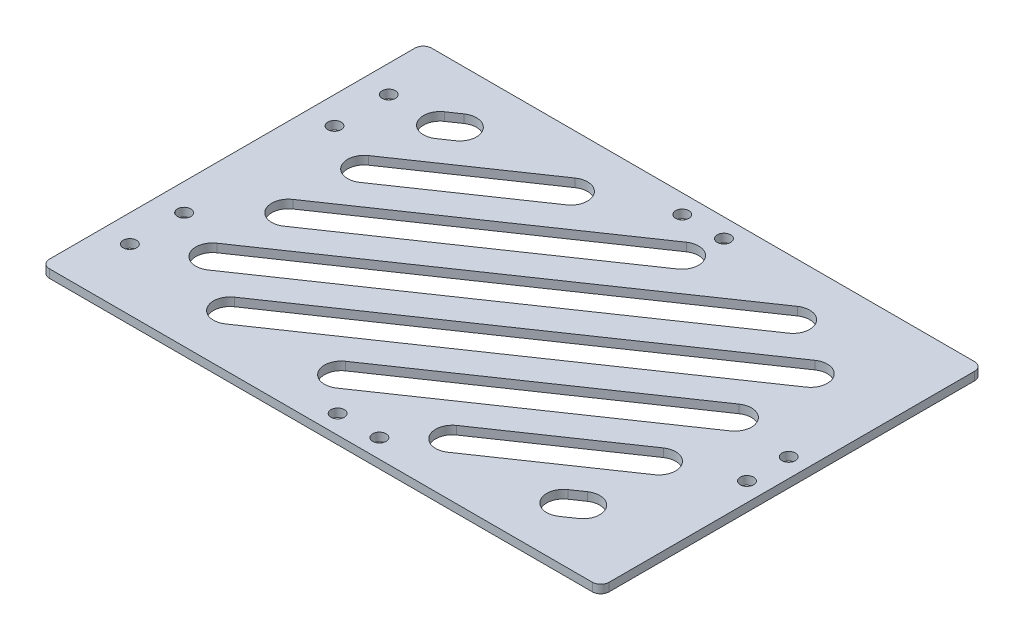
SolidWorks part; units mm, degrees
material "Thornel Mat VMA"
ref_plane "前视基准面" through (0, 0, 0) normal (0, 0, 1) x (1, 0, 0)
ref_plane "上视基准面" through (0, 0, 0) normal (0, 1, 0) x (1, 0, 0)
ref_plane "右视基准面" through (0, 0, 0) normal (1, 0, 0) x (0, 0, -1)
sketch "草图1" plane through (0, 0, 0) normal (0, 1, 0) x (1, 0, 0)
  line L0 (-66, 0) -> (68, 0) construction
  line L1 (-66, 45.75) -> (68, 45.75)
  line L2 (-66, 45.75) -> (-66, -45.75)
  line L3 (-66, -45.75) -> (68, -45.75)
  line L4 (68, 45.75) -> (68, -45.75)
  line L5 (0, 45.75) -> (0, -45.75) construction
  line L6 (-59.5, 31) -> (-59.5, 18) construction
  line L7 (-59.5, -31) -> (-59.5, -18) construction
  line L9 (63.5, 3.75) -> (63.5, -6.25) construction
  line L11 (0.5, -41.25) -> (10.5, -41.25) construction
  line L12 (0.5, 41.25) -> (10.5, 41.25) construction
  circle A0 centre (-59.5, 31) radius 1.6
  circle A1 centre (-59.5, 18) radius 1.6
  circle A2 centre (-59.5, -18) radius 1.6
  circle A3 centre (-59.5, -31) radius 1.6
  circle A6 centre (63.5, 3.75) radius 1.6
  circle A7 centre (63.5, -6.25) radius 1.6
  circle A10 centre (0.5, -41.25) radius 1.6
  circle A11 centre (10.5, -41.25) radius 1.6
  circle A12 centre (10.5, 41.25) radius 1.6
  circle A13 centre (0.5, 41.25) radius 1.6
  point P10 (-66, 0)
  dimension "D1" = 3.2
  dimension "D8" = 4.5
  dimension "D9" = 10
  dimension "D12" = 4.5
  dimension "D10" = 3.2
  dimension "D2" = 13
  dimension "D3" = 68
  dimension "D4" = 66
  dimension "D5" = 91.5
  dimension "D6" = 36
  dimension "D7" = 6.5
  dimension "D11" = 39.5
  dimension "D15" = 57.5
extrude "凸台-拉伸1" add sketch "草图1" along normal blind 2
sketch "队徽" [suppressed] plane through (0, 2, 0) normal (0, 1, 0) x (1, 0, 0)
  line L0 (-25, 38) -> (-25, -22) construction
  line L1 (-12.515, 33.7) -> (-12.515, 35.2787)
  line L2 (-37.485, 33.7) -> (-37.485, 35.2787)
  line L3 (-33.13, 16.8019) -> (-33.13, 11.5819)
  line L4 (-33.13, 11.5819) -> (-34.702, 9.9305)
  line L5 (-34.702, 9.9305) -> (-36.3011, 4.7584)
  line L6 (-33.4579, 3.2225) -> (-31.1856, 10.5724)
  line L7 (-16.5421, 3.2225) -> (-18.8144, 10.5724)
  line L8 (-17.5104, 17.0865) -> (-13.6989, 4.7584)
  line L9 (-21.0663, 32.392) -> (-19.6973, 32.769)
  line L10 (-19.6973, 32.769) -> (-18.0096, 33.5704)
  line L11 (-18.0096, 33.5704) -> (-17.8613, 32.2487)
  line L12 (-18.4024, 35.9034) -> (-17.7524, 35.7605)
  line L13 (-6.1254, -12) -> (-2.6393, -12)
  line L14 (-43.8746, -12) -> (-47.3607, -12)
  arc A0 (-16.6314, -20.8091) -> (-2.6393, -12) centre (-25, 8) ccw
  arc A2 (-33.3686, -20.8091) -> (-33.13, 16.8019) centre (-24.3625, -2.06) cw
  arc A3 (-16.6314, -20.8091) -> (-17.5104, 17.0865) centre (-25.6375, -2.06) ccw
  arc A4 (-19.8705, 26.2753) -> (-12.515, 33.7) centre (-19.94, 33.7) ccw
  arc A5 (-30.1295, 26.2753) -> (-37.485, 33.7) centre (-30.06, 33.7) cw
  arc A6 (-47.3607, -12) -> (-33.3686, -20.8091) centre (-25, 8) ccw
  arc A7 (-36.3011, 4.7584) -> (-33.4579, 3.2225) centre (-25, 22.28) ccw
  arc A9 (-32.1188, 2.6829) -> (-31.1856, 10.5724) centre (-66.67, 10.77) ccw
  arc A10 (-32.1188, 2.6829) -> (-29.0372, 1.8246) centre (-25, 22.28) ccw
  arc A12 (-27.4096, 1.5697) -> (-27.9405, 8.9327) centre (-66.67, 2.44) ccw
  arc A13 (-29.0372, 1.8246) -> (-27.9405, 8.9327) centre (-66.67, 11.27) ccw
  arc A14 (-27.4096, 1.5697) -> (-22.5904, 1.5697) centre (-25, 22.28) ccw
  arc A15 (-22.5904, 1.5697) -> (-22.0595, 8.9327) centre (16.67, 2.44) cw
  arc A16 (-20.9628, 1.8246) -> (-22.0595, 8.9327) centre (16.67, 11.27) cw
  arc A17 (-30.1295, 26.2753) -> (-28.9744, 32.0412) centre (-66.7, 36.6) ccw
  arc A18 (-17.8812, 2.6829) -> (-18.8144, 10.5724) centre (16.67, 10.77) cw
  arc A19 (-19.8705, 26.2753) -> (-21.0663, 32.392) centre (16.7, 36.6) cw
  arc A20 (-20.9628, 1.8246) -> (-17.8812, 2.6829) centre (-25, 22.28) ccw
  arc A21 (-16.5421, 3.2225) -> (-13.6989, 4.7584) centre (-25, 22.28) ccw
  arc A22 (-20.8, 36.4498) -> (-31.4255, 34.2262) centre (-21.93, 15.35) ccw
  arc A23 (-16.5042, 35.0804) -> (-17.7524, 35.7605) centre (-18.3, 33.27) ccw
  arc A25 (-17.8613, 32.2487) -> (-16.5042, 35.0804) centre (-18.3, 34.2) ccw
  arc A29 (-6.1077, 27.9833) -> (-12.515, 35.2787) centre (-17.46, 24.4743) ccw
  arc A30 (-2.2672, 23.4748) -> (-0.7491, 25.6605) centre (-25, 40.8837) ccw
  arc A31 (-6.1077, 27.9833) -> (-5.5019, 30.7996) centre (-25, 33.5203) ccw
  arc A32 (-2.2672, 23.4748) -> (-5.5019, 30.7996) centre (-11.5161, 23.767) ccw
  arc A33 (1.6644, 14.7277) -> (3.8374, 16.2708) centre (-25, 54.5789) ccw
  arc A34 (1.6644, 14.7277) -> (-0.7491, 25.6605) centre (-12.0455, 17.434) ccw
  arc A35 (2.163, 3.7077) -> (4.8783, 5.3) centre (-25, 53.1378) ccw
  arc A36 (2.163, 3.7077) -> (3.8374, 16.2708) centre (-11.3811, 11.906) ccw
  arc A37 (-1.1678, -5.7213) -> (1.8513, -5.3793) centre (-25, 218.1341) ccw
  arc A38 (-1.1678, -5.7213) -> (4.8783, 5.3) centre (-10.7675, 6.7139) ccw
  arc A40 (-6.1254, -12) -> (1.8513, -5.3793) centre (-9.635, 0.344) ccw
  circle A41 centre (-25, 8) radius 27.5 construction
  arc A42 (-43.8923, 27.9833) -> (-44.4981, 30.7996) centre (-25, 33.5203) cw
  arc A43 (-43.8923, 27.9833) -> (-37.485, 35.2787) centre (-32.54, 24.4743) cw
  arc A44 (-47.7328, 23.4748) -> (-44.4981, 30.7996) centre (-38.4839, 23.767) cw
  arc A45 (-47.7328, 23.4748) -> (-49.2509, 25.6605) centre (-25, 40.8837) cw
  arc A46 (-51.6644, 14.7277) -> (-49.2509, 25.6605) centre (-37.9545, 17.434) cw
  arc A47 (-51.6644, 14.7277) -> (-53.8374, 16.2708) centre (-25, 54.5789) cw
  arc A48 (-52.163, 3.7077) -> (-53.8374, 16.2708) centre (-38.6189, 11.906) cw
  arc A49 (-52.163, 3.7077) -> (-54.8783, 5.3) centre (-25, 53.1378) cw
  arc A50 (-48.8322, -5.7213) -> (-54.8783, 5.3) centre (-39.2325, 6.7139) cw
  arc A51 (-48.8322, -5.7213) -> (-51.8513, -5.3793) centre (-25, 218.1341) cw
  arc A52 (-43.8746, -12) -> (-51.8513, -5.3793) centre (-40.365, 0.344) cw
  arc A53 (-28.9744, 32.0412) -> (-31.4255, 34.2262) centre (-30.96, 32.2812) ccw
  spline S0 degree 3 poles (-20.8, 36.4498) (-20.2858, 35.8279) (-18.8685, 36.0059) (-18.4024, 35.9034) knots 0 0 0 0 1 1 1 1
  spline S1 degree 3 poles (-22.2858, 34.0584) (-22.7796, 35.9592) (-21.5435, 34.6039) (-20.1915, 35.1653) (-20.9556, 33.6368) (-22.2858, 34.0584) (-22.7796, 35.9592) (-21.5435, 34.6039) knots -0.60913 -0.442651 -0.194324 0 0.241967 0.39087 0.557349 0.805676 1 1.241967 1.39087 1.557349 only from (-22.5, 35.3861) to (-22.5, 35.3861)
  dimension "D1" = 60
  dimension "D2" = 20.8
  dimension "D5" = 25.7
  dimension "D7" = 7.425
  dimension "D8" = 41.7
  dimension "D16" = 35.485
  dimension "D19" = 39.27
  dimension "D21" = 0.5
  dimension "D22" = 38.8
  dimension "D23" = 41.7
  dimension "D25" = 55
  dimension "D26" = 7.35
  dimension "D28" = 21.13
  dimension "D29" = 25.27
  dimension "D31" = 0.93
  dimension "D32" = 2
  dimension "D33" = 5.1
  dimension "D41" = 8
  dimension "D42" = 9.59
  dimension "D44" = 7
  dimension "D46" = 10
  dimension "D48" = 20
  dimension "D49" = 11.1
  dimension "D43" = 11.02
  dimension "D47" = 8
  dimension "D52" = 38
  dimension "D57" = 2
  dimension "D3" = 10.06
  dimension "D4" = 1.275
  dimension "D6" = 10.12
  dimension "D9" = 14.28
  dimension "D10" = 8.13
  dimension "D11" = 5.22
  dimension "D12" = 136.41
  dimension "D13" = 2.28
  dimension "D14" = 17.18
  dimension "D15" = 3.17
  dimension "D17" = 41.67
  dimension "D18" = 2.77
  dimension "D20" = 8.33
  dimension "D24" = 28.6
  dimension "D27" = 3.07
  dimension "D30" = 6.7
  dimension "D34" = 74.6
  dimension "D35" = 1.42
  dimension "D36" = 170
  dimension "D37" = 71
  dimension "D38" = 1.33
  dimension "D39" = 0.65
  dimension "D40" = 77.6
  dimension "D45" = 7.54
  dimension "D50" = 11.02
  dimension "D51" = 10.45
  dimension "D53" = 4.8
  dimension "D54" = 28.5
  dimension "D55" = 4.2
  dimension "D56" = 90
  dimension "D58" = 5.96
  dimension "D59" = 2.5
  dimension "D60" = 2
  dimension "D61" = 0.5
  dimension "D62" = 1.2
  dimension "D63" = 0.3
  dimension "D64" = 0.4
  dimension "D65" = 1
  dimension "D66" = 0.8
  dimension "D67" = 8
  dimension "D68" = 25
sketch "草图4" [suppressed] plane through (0, 2, 0) normal (0, 1, 0) x (1, 0, 0)
  line L0 (-25, 42) -> (-25, -26) construction
  line L3 (-27.5, 41.908) -> (-27.5, 35.7326)
  line L8 (-22.5, 41.908) -> (-22.5, 36.4723)
  line L9 (6.4758, 20.8558) -> (1.7989, 19.3361)
  line L10 (8.0209, 16.1005) -> (4.1747, 14.8508)
  line L11 (-3.0469, -17.9627) -> (-5.4052, -14.7166)
  line L12 (-7.0919, -20.9016) -> (-9.4503, -17.6556)
  line L13 (-42.9081, -20.9016) -> (-40.5497, -17.6556)
  line L42 (-46.9531, -17.9627) -> (-44.5948, -14.7166)
  line L43 (-58.0209, 16.1005) -> (-54.1747, 14.8508)
  line L44 (-56.4758, 20.8558) -> (-51.7989, 19.3361)
  line L45 (-43.3105, 6.5198) -> (-49.4142, 0.4161)
  line L46 (-44.7, 2.3019) -> (-48, -0.9981)
  line L48 (-43.8746, -12) -> (-47.3607, -12)
  line L49 (-33.13, 16.8019) -> (-33.13, 11.5819)
  line L50 (-33.13, 11.5819) -> (-34.702, 9.9305)
  line L51 (-34.702, 9.9305) -> (-36.3011, 4.7584)
  line L52 (-33.4579, 3.2225) -> (-31.1856, 10.5724)
  line L53 (-18.8144, 10.5724) -> (-16.5421, 3.2225)
  line L54 (-13.6989, 4.7584) -> (-17.5104, 17.0865)
  line L55 (-2.6393, -12) -> (-6.1254, -12)
  line L56 (-12.515, 35.2787) -> (-12.515, 33.7)
  line L57 (-21.0663, 32.392) -> (-19.6973, 32.769)
  line L58 (-19.6973, 32.769) -> (-18.0096, 33.5704)
  line L59 (-18.0096, 33.5704) -> (-17.8613, 32.2487)
  line L60 (-17.7524, 35.7605) -> (-18.4024, 35.9034)
  line L61 (-37.485, 33.7) -> (-37.485, 35.2787)
  line L62 (-43.8746, -12) -> (-47.3607, -12)
  line L63 (-33.13, 16.8019) -> (-33.13, 11.5819)
  line L64 (-33.13, 11.5819) -> (-34.702, 9.9305)
  line L65 (-34.702, 9.9305) -> (-36.3011, 4.7584)
  line L66 (-33.4579, 3.2225) -> (-31.1856, 10.5724)
  line L67 (-18.8144, 10.5724) -> (-16.5421, 3.2225)
  line L68 (-13.6989, 4.7584) -> (-17.5104, 17.0865)
  line L69 (-2.6393, -12) -> (-6.1254, -12)
  line L70 (-12.515, 35.2787) -> (-12.515, 33.7)
  line L71 (-21.0663, 32.392) -> (-19.6973, 32.769)
  line L72 (-19.6973, 32.769) -> (-18.0096, 33.5704)
  line L73 (-18.0096, 33.5704) -> (-17.8613, 32.2487)
  line L74 (-17.7524, 35.7605) -> (-18.4024, 35.9034)
  line L75 (-37.485, 33.7) -> (-37.485, 35.2787)
  line L77 (-49.4142, 0.4161) -> (-48, -0.9981)
  line L78 (-44.8311, 21.2627) -> (-36.3458, 29.7479) construction
  line L79 (-54.0846, 8.5198) -> (-50.5029, 8.5198)
  line L80 (-50.5029, 8.5198) -> (-36.2226, 22.8001)
  line L81 (-53.5066, 6.5198) -> (-49.6745, 6.5198)
  line L82 (-49.6745, 6.5198) -> (-34.8084, 21.3859)
  line L83 (-44.5227, 22.9853) -> (-36.8384, 30.6696)
  line L84 (-43.1085, 21.5711) -> (-35.7499, 28.9297)
  arc A6 (-27.5, 41.908) -> (-56.4758, 20.8558) centre (-25, 8) ccw
  arc A7 (-27.5, 35.7326) -> (-31.4255, 34.2262) centre (-21.93, 15.35) ccw
  arc A8 (-42.9081, -20.9016) -> (-7.0919, -20.9016) centre (-25, 8) ccw
  arc A9 (-40.5497, -17.6556) -> (-33.3686, -20.8091) centre (-25, 8) ccw
  arc A10 (-3.0469, -17.9627) -> (8.0209, 16.1005) centre (-25, 8) ccw
  arc A11 (-5.4052, -14.7166) -> (-2.6393, -12) centre (-25, 8) ccw
  arc A12 (6.4758, 20.8558) -> (-22.5, 41.908) centre (-25, 8) ccw
  arc A13 (-58.0209, 16.1005) -> (-46.9531, -17.9627) centre (-25, 8) ccw
  arc A15 (-44.7, 2.3019) -> (-33.3686, -20.8091) centre (-24.3625, -2.06) ccw
  arc A18 (-34.8084, 21.3859) -> (-36.2226, 22.8001) centre (-34.5, 23.1085) ccw
  arc A19 (-53.5066, 6.5198) -> (-52.163, 3.7077) centre (-38.6189, 11.906) ccw
  arc A20 (-44.5227, 22.9853) -> (-43.1085, 21.5711) centre (-44.8311, 21.2627) ccw
  arc A21 (-35.7499, 28.9297) -> (-30.1295, 26.2753) centre (-30.06, 33.7) ccw
  arc A135 (-47.3607, -12) -> (-33.3686, -20.8091) centre (-25, 8) ccw
  arc A136 (-33.13, 16.8019) -> (-33.3686, -20.8091) centre (-24.3625, -2.06) ccw
  arc A137 (-36.3011, 4.7584) -> (-33.4579, 3.2225) centre (-25, 22.28) ccw
  arc A138 (-32.1188, 2.6829) -> (-31.1856, 10.5724) centre (-66.67, 10.77) ccw
  arc A139 (-32.1188, 2.6829) -> (-29.0372, 1.8246) centre (-25, 22.28) ccw
  arc A140 (-29.0372, 1.8246) -> (-27.9405, 8.9327) centre (-66.67, 11.27) ccw
  arc A141 (-27.4096, 1.5697) -> (-27.9405, 8.9327) centre (-66.67, 2.44) ccw
  arc A142 (-27.4096, 1.5697) -> (-22.5904, 1.5697) centre (-25, 22.28) ccw
  arc A143 (-22.0595, 8.9327) -> (-22.5904, 1.5697) centre (16.67, 2.44) ccw
  arc A144 (-22.0595, 8.9327) -> (-20.9628, 1.8246) centre (16.67, 11.27) ccw
  arc A145 (-20.9628, 1.8246) -> (-17.8812, 2.6829) centre (-25, 22.28) ccw
  arc A146 (-18.8144, 10.5724) -> (-17.8812, 2.6829) centre (16.67, 10.77) ccw
  arc A147 (-16.5421, 3.2225) -> (-13.6989, 4.7584) centre (-25, 22.28) ccw
  arc A148 (-16.6314, -20.8091) -> (-17.5104, 17.0865) centre (-25.6375, -2.06) ccw
  arc A149 (-16.6314, -20.8091) -> (-2.6393, -12) centre (-25, 8) ccw
  arc A150 (-6.1254, -12) -> (1.8513, -5.3793) centre (-9.635, 0.344) ccw
  arc A151 (-1.1678, -5.7213) -> (1.8513, -5.3793) centre (-25, 218.1341) ccw
  arc A152 (-1.1678, -5.7213) -> (4.8783, 5.3) centre (-10.7675, 6.7139) ccw
  arc A153 (2.163, 3.7077) -> (4.8783, 5.3) centre (-25, 53.1378) ccw
  arc A154 (2.163, 3.7077) -> (3.8374, 16.2708) centre (-11.3811, 11.906) ccw
  arc A155 (1.6644, 14.7277) -> (3.8374, 16.2708) centre (-25, 54.5789) ccw
  arc A156 (1.6644, 14.7277) -> (-0.7491, 25.6605) centre (-12.0455, 17.434) ccw
  arc A157 (-2.2672, 23.4748) -> (-0.7491, 25.6605) centre (-25, 40.8837) ccw
  arc A158 (-2.2672, 23.4748) -> (-5.5019, 30.7996) centre (-11.5161, 23.767) ccw
  arc A159 (-6.1077, 27.9833) -> (-5.5019, 30.7996) centre (-25, 33.5203) ccw
  arc A160 (-6.1077, 27.9833) -> (-12.515, 35.2787) centre (-17.46, 24.4743) ccw
  arc A161 (-19.8705, 26.2753) -> (-12.515, 33.7) centre (-19.94, 33.7) ccw
  arc A162 (-21.0663, 32.392) -> (-19.8705, 26.2753) centre (16.7, 36.6) ccw
  arc A163 (-17.8613, 32.2487) -> (-16.5042, 35.0804) centre (-18.3, 34.2) ccw
  arc A164 (-16.5042, 35.0804) -> (-17.7524, 35.7605) centre (-18.3, 33.27) ccw
  arc A165 (-20.8, 36.4498) -> (-31.4255, 34.2262) centre (-21.93, 15.35) ccw
  arc A166 (-30.1295, 26.2753) -> (-28.9744, 32.0412) centre (-66.7, 36.6) ccw
  arc A167 (-37.485, 33.7) -> (-30.1295, 26.2753) centre (-30.06, 33.7) ccw
  arc A168 (-37.485, 35.2787) -> (-43.8923, 27.9833) centre (-32.54, 24.4743) ccw
  arc A169 (-44.4981, 30.7996) -> (-43.8923, 27.9833) centre (-25, 33.5203) ccw
  arc A170 (-44.4981, 30.7996) -> (-47.7328, 23.4748) centre (-38.4839, 23.767) ccw
  arc A171 (-49.2509, 25.6605) -> (-47.7328, 23.4748) centre (-25, 40.8837) ccw
  arc A172 (-49.2509, 25.6605) -> (-51.6644, 14.7277) centre (-37.9545, 17.434) ccw
  arc A173 (-53.8374, 16.2708) -> (-51.6644, 14.7277) centre (-25, 54.5789) ccw
  arc A174 (-53.8374, 16.2708) -> (-52.163, 3.7077) centre (-38.6189, 11.906) ccw
  arc A175 (-54.8783, 5.3) -> (-52.163, 3.7077) centre (-25, 53.1378) ccw
  arc A176 (-54.8783, 5.3) -> (-48.8322, -5.7213) centre (-39.2325, 6.7139) ccw
  arc A177 (-51.8513, -5.3793) -> (-48.8322, -5.7213) centre (-25, 218.1341) ccw
  arc A178 (-51.8513, -5.3793) -> (-43.8746, -12) centre (-40.365, 0.344) ccw
  arc A179 (-47.3607, -12) -> (-44.5948, -14.7166) centre (-25, 8) ccw
  arc A180 (-33.13, 16.8019) -> (-43.3105, 6.5198) centre (-24.3625, -2.06) ccw
  arc A181 (-36.3011, 4.7584) -> (-33.4579, 3.2225) centre (-25, 22.28) ccw
  arc A182 (-32.1188, 2.6829) -> (-31.1856, 10.5724) centre (-66.67, 10.77) ccw
  arc A183 (-32.1188, 2.6829) -> (-29.0372, 1.8246) centre (-25, 22.28) ccw
  arc A184 (-29.0372, 1.8246) -> (-27.9405, 8.9327) centre (-66.67, 11.27) ccw
  arc A185 (-27.4096, 1.5697) -> (-27.9405, 8.9327) centre (-66.67, 2.44) ccw
  arc A186 (-27.4096, 1.5697) -> (-22.5904, 1.5697) centre (-25, 22.28) ccw
  arc A187 (-22.0595, 8.9327) -> (-22.5904, 1.5697) centre (16.67, 2.44) ccw
  arc A188 (-22.0595, 8.9327) -> (-20.9628, 1.8246) centre (16.67, 11.27) ccw
  arc A189 (-20.9628, 1.8246) -> (-17.8812, 2.6829) centre (-25, 22.28) ccw
  arc A190 (-18.8144, 10.5724) -> (-17.8812, 2.6829) centre (16.67, 10.77) ccw
  arc A191 (-16.5421, 3.2225) -> (-13.6989, 4.7584) centre (-25, 22.28) ccw
  arc A192 (-16.6314, -20.8091) -> (-17.5104, 17.0865) centre (-25.6375, -2.06) ccw
  arc A193 (-16.6314, -20.8091) -> (-9.4503, -17.6556) centre (-25, 8) ccw
  arc A194 (-6.1254, -12) -> (1.8513, -5.3793) centre (-9.635, 0.344) ccw
  arc A195 (-1.1678, -5.7213) -> (1.8513, -5.3793) centre (-25, 218.1341) ccw
  arc A196 (-1.1678, -5.7213) -> (4.8783, 5.3) centre (-10.7675, 6.7139) ccw
  arc A197 (2.163, 3.7077) -> (4.8783, 5.3) centre (-25, 53.1378) ccw
  arc A198 (2.163, 3.7077) -> (4.1747, 14.8508) centre (-11.3811, 11.906) ccw
  arc A200 (1.7989, 19.3361) -> (-0.7491, 25.6605) centre (-12.0455, 17.434) ccw
  arc A201 (-2.2672, 23.4748) -> (-0.7491, 25.6605) centre (-25, 40.8837) ccw
  arc A202 (-2.2672, 23.4748) -> (-5.5019, 30.7996) centre (-11.5161, 23.767) ccw
  arc A203 (-6.1077, 27.9833) -> (-5.5019, 30.7996) centre (-25, 33.5203) ccw
  arc A204 (-6.1077, 27.9833) -> (-12.515, 35.2787) centre (-17.46, 24.4743) ccw
  arc A205 (-19.8705, 26.2753) -> (-12.515, 33.7) centre (-19.94, 33.7) ccw
  arc A206 (-21.0663, 32.392) -> (-19.8705, 26.2753) centre (16.7, 36.6) ccw
  arc A207 (-17.8613, 32.2487) -> (-16.5042, 35.0804) centre (-18.3, 34.2) ccw
  arc A208 (-16.5042, 35.0804) -> (-17.7524, 35.7605) centre (-18.3, 33.27) ccw
  arc A209 (-20.8, 36.4498) -> (-22.5, 36.4723) centre (-21.93, 15.35) ccw
  arc A210 (-30.1295, 26.2753) -> (-28.9744, 32.0412) centre (-66.7, 36.6) ccw
  arc A211 (-37.485, 33.7) -> (-36.8384, 30.6696) centre (-30.06, 33.7) ccw
  arc A212 (-37.485, 35.2787) -> (-43.8923, 27.9833) centre (-32.54, 24.4743) ccw
  arc A213 (-44.4981, 30.7996) -> (-43.8923, 27.9833) centre (-25, 33.5203) ccw
  arc A214 (-44.4981, 30.7996) -> (-47.7328, 23.4748) centre (-38.4839, 23.767) ccw
  arc A215 (-49.2509, 25.6605) -> (-47.7328, 23.4748) centre (-25, 40.8837) ccw
  arc A216 (-49.2509, 25.6605) -> (-51.7989, 19.3361) centre (-37.9545, 17.434) ccw
  arc A218 (-54.1747, 14.8508) -> (-54.0846, 8.5198) centre (-38.6189, 11.906) ccw
  arc A219 (-54.8783, 5.3) -> (-52.163, 3.7077) centre (-25, 53.1378) ccw
  arc A220 (-54.8783, 5.3) -> (-48.8322, -5.7213) centre (-39.2325, 6.7139) ccw
  arc A221 (-51.8513, -5.3793) -> (-48.8322, -5.7213) centre (-25, 218.1341) ccw
  arc A222 (-51.8513, -5.3793) -> (-43.8746, -12) centre (-40.365, 0.344) ccw
  arc A232 (-28.9744, 32.0412) -> (-31.4255, 34.2262) centre (-30.96, 32.2812) ccw
  arc A233 (-28.9744, 32.0412) -> (-31.4255, 34.2262) centre (-30.96, 32.2812) ccw
  spline S0 degree 3 poles (-21.5435, 34.6039) (-22.7796, 35.9592) (-22.2858, 34.0584) (-20.9556, 33.6368) (-20.1915, 35.1653) (-21.5435, 34.6039) (-22.7796, 35.9592) (-22.2858, 34.0584) knots -0.557349 -0.39087 -0.241967 0 0.194324 0.442651 0.60913 0.758033 1 1.194324 1.442651 1.60913 only from (-22.5, 35.3861) to (-22.5, 35.3861) construction
  spline S1 degree 3 poles (-1772.4748, -924.8076) (1747.4533, 1033.1302) (-1763.0741, -1000.2366) (1663.8646, 1113.8816) knots -9.353839 -9.353839 -9.353839 -9.353839 10.249272 10.249272 10.249272 10.249272 only from (-18.4024, 35.9034) to (-20.8, 36.4498)
  spline S2 degree 3 poles (-18.4024, 35.9034) (-18.8685, 36.0059) (-20.2858, 35.8279) (-20.8, 36.4498) knots 0 0 0 0 1 1 1 1
  spline S3 degree 3 poles (-21.5435, 34.6039) (-22.7796, 35.9592) (-22.2858, 34.0584) (-20.9556, 33.6368) (-20.1915, 35.1653) (-21.5435, 34.6039) (-22.7796, 35.9592) (-22.2858, 34.0584) knots -0.557349 -0.39087 -0.241967 0 0.194324 0.442651 0.60913 0.758033 1 1.194324 1.442651 1.60913 only from (-22.5, 35.3861) to (-22.5, 35.3861)
  point P86 (-25, 8)
  dimension "D2" = 4
  dimension "D4" = 5
  dimension "D5" = 1.75
  dimension "D8" = 2
  dimension "D12" = 2
  dimension "D14" = 1
  dimension "D3" = 5
  dimension "D6" = 2
  dimension "D7" = 45
  dimension "D9" = 4
  dimension "D10" = 19.7
  dimension "D11" = 23
  dimension "D13" = 2
  dimension "D15" = 12
  dimension "D16" = 9.5
  dimension "D17" = 4.5
  dimension "D21" = 8
  dimension "D1" = 0
extrude "切除-拉伸1" [suppressed] cut sketch "草图4" against normal through all contours A210 A233 A7 L3 A6 L44 A216 A215 A214 A213 A212 L75 A211 | S2 L74 A208 A207 L73 L72 L71 A206 A205 L70 A204 A203 A202 A201 A200 L9 A12 L8 A209 | A222 A221 A220 A219 A218 L43 A13 L42 A179 L62 | L0 A186 A185 A184 A183 A182 L66 A181 L65 L64 L63 A180 A9 L13 A8 | A186 L0 A8 L12 A193 A192 L68 A191 L67 A190 A189 A188 A187 | A198 A197 A196 A195 A194 L69 A11 L11 A10 L10 | S3
fillet "R0.5 圆角1" [suppressed] radius 0.5
fillet "R0.5 圆角2" [suppressed] radius 0.5
fillet "R2 圆角3" [suppressed] radius 2
sketch "草图5" plane through (0, 2, 0) normal (0, 1, 0) x (1, 0, 0)
  line L0 (-66, -45.75) -> (68, 45.75) construction
  line L1 (-47, 30.7958) -> (-44.2163, 32.6966) construction
  line L2 (-49.2556, 34.0992) -> (-46.472, 36)
  line L3 (-44.7444, 27.4925) -> (-41.9607, 29.3933)
  line L4 (-47, 12.6324) -> (-17.6163, 32.6966) construction
  line L5 (-49.2556, 15.9358) -> (-19.872, 36)
  line L6 (-44.7444, 9.3291) -> (-15.3607, 29.3933)
  line L7 (-47, -5.531) -> (8.9836, 32.6966) construction
  line L8 (-49.2556, -2.2277) -> (6.728, 36)
  line L9 (-44.7444, -8.8343) -> (11.2393, 29.3933)
  line L10 (-47, -23.6944) -> (35.5836, 32.6966) construction
  line L11 (-49.2556, -20.3911) -> (33.328, 36)
  line L12 (-44.7444, -26.9978) -> (37.8392, 29.3933)
  line L13 (-33.7, -32.7761) -> (48.8836, 23.6149) construction
  line L14 (-66.1164, 45.75) -> (68, -45.8295) construction
  line L15 (-35.9557, -29.4728) -> (46.6279, 26.9183)
  line L16 (-31.4444, -36.0795) -> (51.1392, 20.3116)
  line L17 (-7.1, -32.7761) -> (48.8836, 5.4515) construction
  line L18 (-9.3557, -29.4728) -> (46.6279, 8.7549)
  line L19 (-4.8444, -36.0795) -> (51.1392, 2.1482)
  line L20 (19.4999, -32.7761) -> (48.8836, -12.7119) construction
  line L21 (17.2443, -29.4728) -> (46.6279, -9.4086)
  line L22 (21.7556, -36.0795) -> (51.1392, -16.0153)
  line L23 (46.0999, -32.7761) -> (48.8836, -30.8753) construction
  line L24 (43.8443, -29.4728) -> (46.6279, -27.572)
  line L25 (48.3555, -36.0795) -> (51.1392, -34.1787)
  line L26 (-66, 45.75) -> (68, -45.75) construction
  line L27 (68, 45.75) -> (-66, 45.75) construction
  line L28 (68, -45.75) -> (68, 45.75) construction
  arc A0 (-49.2556, 34.0992) -> (-44.7444, 27.4925) centre (-47, 30.7958) ccw
  arc A1 (-41.9607, 29.3933) -> (-46.472, 36) centre (-44.2163, 32.6966) ccw
  arc A2 (-49.2556, 15.9358) -> (-44.7444, 9.3291) centre (-47, 12.6324) ccw
  arc A3 (-15.3607, 29.3933) -> (-19.872, 36) centre (-17.6163, 32.6966) ccw
  arc A4 (-49.2556, -2.2277) -> (-44.7444, -8.8343) centre (-47, -5.531) ccw
  arc A5 (11.2393, 29.3933) -> (6.728, 36) centre (8.9836, 32.6966) ccw
  arc A6 (-49.2556, -20.3911) -> (-44.7444, -26.9978) centre (-47, -23.6944) ccw
  arc A7 (37.8392, 29.3933) -> (33.328, 36) centre (35.5836, 32.6966) ccw
  arc A8 (-35.9557, -29.4728) -> (-31.4444, -36.0795) centre (-33.7, -32.7761) ccw
  arc A9 (51.1392, 20.3116) -> (46.6279, 26.9183) centre (48.8836, 23.6149) ccw
  arc A10 (-9.3557, -29.4728) -> (-4.8444, -36.0795) centre (-7.1, -32.7761) ccw
  arc A11 (51.1392, 2.1482) -> (46.6279, 8.7549) centre (48.8836, 5.4515) ccw
  arc A12 (17.2443, -29.4728) -> (21.7556, -36.0795) centre (19.4999, -32.7761) ccw
  arc A13 (51.1392, -16.0153) -> (46.6279, -9.4086) centre (48.8836, -12.7119) ccw
  arc A14 (43.8443, -29.4728) -> (48.3555, -36.0795) centre (46.0999, -32.7761) ccw
  arc A15 (51.1392, -34.1787) -> (46.6279, -27.572) centre (48.8836, -30.8753) ccw
  circle A16 centre (-59.5, -18) radius 1.6 construction
  point P6 (-45.6082, 31.7462)
  point P12 (-32.3082, 22.6645)
  point P19 (-19.0082, 13.5828)
  point P26 (-5.7082, 4.5011)
  point P33 (7.5918, -4.5806)
  point P44 (20.8918, -13.6623)
  point P51 (34.1918, -22.744)
  point P58 (47.4917, -31.8257)
  point P64 (-61.0403, 45.75)
  point P67 (68, -42.3496)
  dimension "D1" = 4
  dimension "D2" = 7
  dimension "D3" = 3.5
  dimension "D4" = 7
  dimension "D5" = 7
  dimension "D6" = 7
  dimension "D7" = 7
  dimension "D8" = 7
  dimension "D9" = 7
  dimension "D10" = 100
  dimension "D11" = 12.5
extrude "切除-拉伸2" cut sketch "草图5" against normal through all and the other way through all
fillet "R2 圆角1" radius 2 4 edges at (-66, 1, -45.75) (68, 1, -45.75) (68, 1, 45.75) (-66, 1, 45.75)
